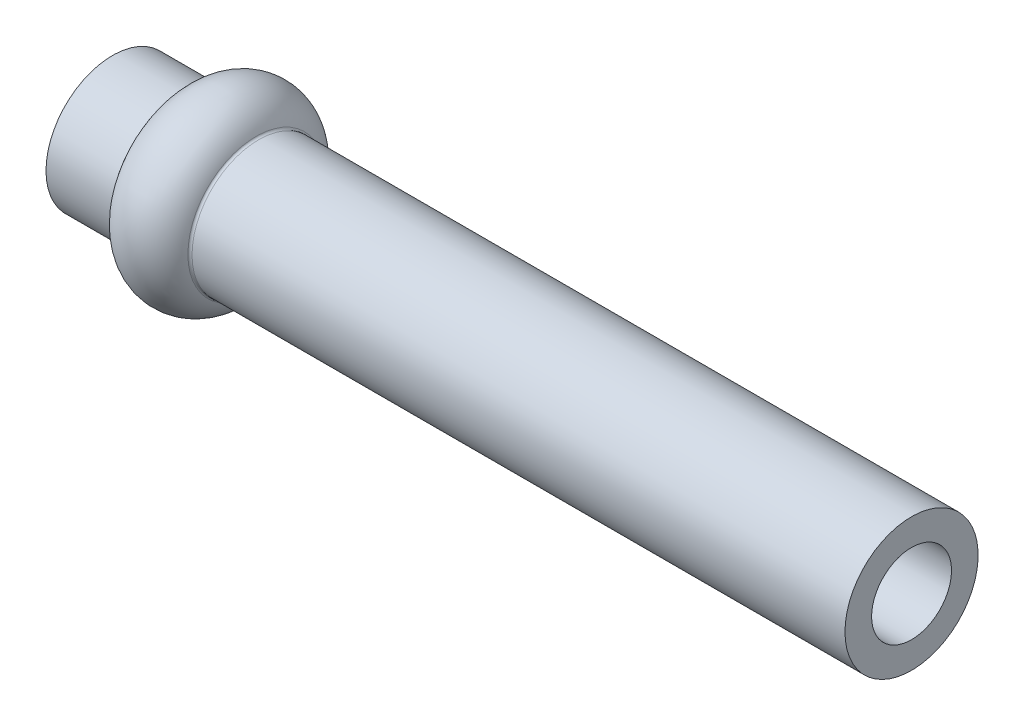
SolidWorks part; units mm, degrees
material "10#"
ref_plane "Front Plane" through (0, 0, 0) normal (0, 0, 1) x (1, 0, 0)
ref_plane "Top Plane" through (0, 0, 0) normal (0, 1, 0) x (1, 0, 0)
ref_plane "Right Plane" through (0, 0, 0) normal (1, 0, 0) x (0, 0, -1)
sketch "Sketch1" plane through (0, 0, 0) normal (0, 0, 1) x (1, 0, 0)
  line L0 (0, 0) -> (32.8973, 0) construction
  line L1 (0, 2.5) -> (2.5858, 2.5)
  line L2 (30, 2.5) -> (30, 1.5)
  line L3 (30, 1.5) -> (0, 1.5)
  line L4 (0, 1.5) -> (0, 2.5)
  line L5 (5.4142, 2.5) -> (30, 2.5)
  arc A0 (5.4142, 2.5) -> (2.5858, 2.5) centre (4, 2) ccw
  dimension "D6" = 3
  dimension "D1" = 1.5
  dimension "D2" = 1
  dimension "D3" = 30
  dimension "D4" = 0.5
  dimension "D5" = 4
revolve "Revolve1" add sketch "Sketch1" angle 360 about L0
fillet "Fillet1" radius 0.1 2 edges at (5.4142, 0, 2.5) (2.5858, 0, 2.5)
